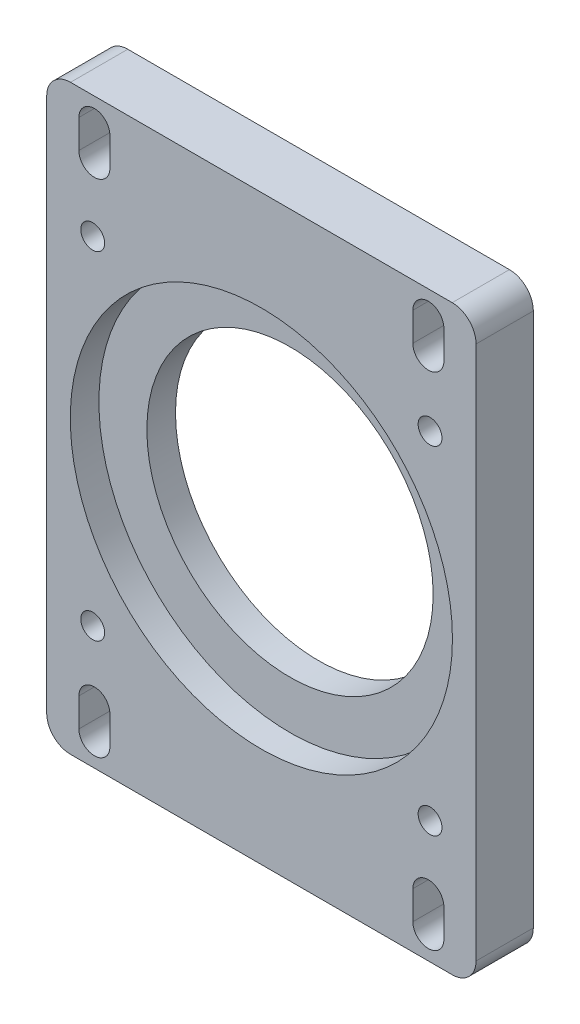
SolidWorks part; units mm, degrees
material "45"
ref_plane "Front Plane" through (0, 0, 0) normal (0, 0, 1) x (1, 0, 0)
ref_plane "Top Plane" through (0, 0, 0) normal (0, 1, 0) x (1, 0, 0)
ref_plane "Right Plane" through (0, 0, 0) normal (1, 0, 0) x (0, 0, -1)
sketch "Sketch1" plane through (0, 0, 0) normal (0, 0, 1) x (1, 0, 0)
  line L1 (-45, 61) -> (45, 61)
  line L2 (-45, 61) -> (-45, -61)
  line L3 (-45, -61) -> (45, -61)
  line L4 (45, 61) -> (45, -61)
  line L5 (-45, 61) -> (45, -61) construction
  line L6 (-45, -61) -> (45, 61) construction
  point P0 (0, 0)
  dimension "D1" = 90
  dimension "D2" = 122
extrude "Boss-Extrude1" add sketch "Sketch1" along normal blind 12
sketch "Sketch2" plane through (0, 0, 12) normal (0, 0, 1) x (1, 0, 0)
  circle A0 centre (0, 0) radius 30
  dimension "D1" = 60
extrude "Cut-Extrude1" cut sketch "Sketch2" against normal through all
sketch "Sketch3" plane through (0, 0, 12) normal (0, 0, 1) x (1, 0, 0)
  circle A0 centre (0, 0) radius 40.05
  dimension "D1" = 80.1
extrude "Cut-Extrude2" cut sketch "Sketch3" against normal blind 6
hole_wizard "M6 Tapped Hole1" positions "Sketch4" profile "Sketch5" tap size "M6" standard "GB" end condition through all
sketch "Sketch4" plane through (0, 0, 12) normal (0, 0, 1) x (1, 0, 0)
  line L1 (-35.3553, 35.3553) -> (35.3553, 35.3553)
  line L2 (-35.3553, 35.3553) -> (-35.3553, -35.3553)
  line L3 (-35.3553, -35.3553) -> (35.3553, -35.3553)
  line L4 (35.3553, 35.3553) -> (35.3553, -35.3553)
  line L5 (-35.3553, 35.3553) -> (35.3553, -35.3553) construction
  line L6 (-35.3553, -35.3553) -> (35.3553, 35.3553) construction
  circle A0 centre (0, 0) radius 50
  point P0 (35.3553, 35.3553)
  point P2 (-35.3553, 35.3553)
  point P4 (-35.3553, -35.3553)
  point P6 (35.3553, -35.3553)
  dimension "D1" = 100
sketch "Sketch5" plane through (35.3553, 35.3553, 12) normal (1, 0, 0) x (0, -1, 0)
  line L0 (0, 0) -> (0, 12)
  line L1 (0, 12) -> (2.5, 12)
  line L2 (2.5, 12) -> (2.5, 0)
  line L5 (2.5, 0) -> (0, 0)
  line L11 (0, -6.35) -> (0, 107.95) construction
  dimension "通孔螺纹孔钻头直径" = 5
  dimension "通孔螺纹孔钻头深度" = 12
cosmetic thread "Hole Cosmetic Thread1" parameters "D2"=6
cosmetic thread "Hole Cosmetic Thread2" parameters "D2"=6
cosmetic thread "Hole Cosmetic Thread3" parameters "D2"=6
cosmetic thread "Hole Cosmetic Thread4" parameters "D2"=6
sketch "Sketch6" plane through (0, 0, 12) normal (0, 0, 1) x (1, 0, 0)
  line L0 (-35, 55.5) -> (-35, 49.5) construction
  line L1 (-31.75, 55.5) -> (-31.75, 49.5)
  line L2 (-38.25, 55.5) -> (-38.25, 49.5)
  line L3 (-80.4589, 0) -> (103.2741, 0)
  line L4 (0, 81.6607) -> (0, -95.879)
  line L5 (35, 55.5) -> (35, 49.5) construction
  line L6 (31.75, 55.5) -> (31.75, 49.5)
  line L7 (38.25, 55.5) -> (38.25, 49.5)
  line L8 (35, -55.5) -> (35, -49.5) construction
  line L9 (31.75, -55.5) -> (31.75, -49.5)
  line L10 (38.25, -55.5) -> (38.25, -49.5)
  line L11 (-35, -55.5) -> (-35, -49.5) construction
  line L12 (-31.75, -55.5) -> (-31.75, -49.5)
  line L13 (-38.25, -55.5) -> (-38.25, -49.5)
  arc A0 (-31.75, 55.5) -> (-38.25, 55.5) centre (-35, 55.5) ccw
  arc A1 (-38.25, 49.5) -> (-31.75, 49.5) centre (-35, 49.5) ccw
  arc A2 (31.75, 55.5) -> (38.25, 55.5) centre (35, 55.5) cw
  arc A3 (38.25, 49.5) -> (31.75, 49.5) centre (35, 49.5) cw
  arc A4 (31.75, -55.5) -> (38.25, -55.5) centre (35, -55.5) ccw
  arc A5 (38.25, -49.5) -> (31.75, -49.5) centre (35, -49.5) ccw
  arc A6 (-31.75, -55.5) -> (-38.25, -55.5) centre (-35, -55.5) cw
  arc A7 (-38.25, -49.5) -> (-31.75, -49.5) centre (-35, -49.5) cw
  point P2 (-35, 52.5)
  point P14 (35, 52.5)
  point P21 (35, -52.5)
  point P28 (-35, -52.5)
  dimension "D1" = 6
  dimension "D2" = 35
  dimension "D3" = 49.5
  dimension "D4" = 6.5
extrude "Cut-Extrude3" cut sketch "Sketch6" against normal through all contours L2 A1 L1 A0 | A3 L7 A2 L6 | L10 A5 L9 A4 | A7 L13 A6 L12
fillet "Fillet1" radius 5 4 edges at (-45, 61, 6) (45, 61, 6) (-45, -61, 6) (45, -61, 6)
